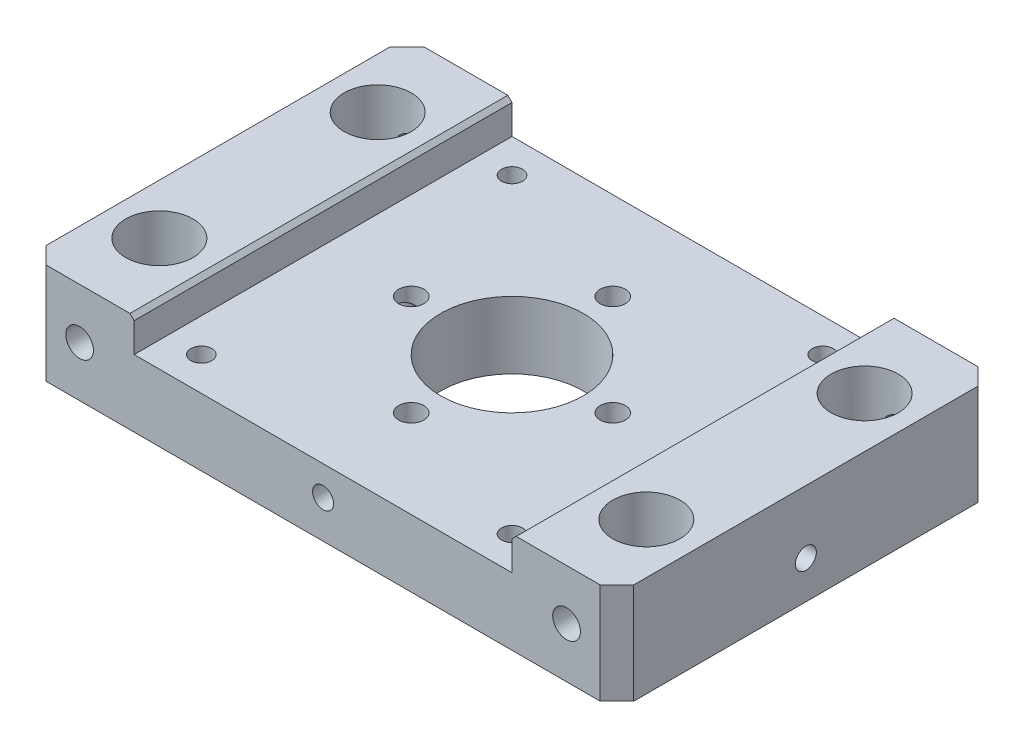
from build123d import *

# Parameters (mm, degrees)
SKETCH1_W                       = 70
SKETCH1_H                       = 45
BOSS_EXTRUDE1_DEPTH             = 12
SKETCH2_W                       = 45
SKETCH2_H                       = 45
CUT_EXTRUDE1_DEPTH              = 4
SKETCH3_R                       = 4
CUT_EXTRUDE2_DEPTH              = 50
SKETCH4_R                       = 8.5
CUT_EXTRUDE3_DEPTH              = 50
SKETCH5_R                       = 0.5
CUT_EXTRUDE4_DEPTH              = 7
M4_TAPPED_HOLE1_AT_2_COUNT      = 2
M4_TAPPED_HOLE1_AT_2_PITCH      = 58
SKETCH7_R                       = 1.5
CUT_EXTRUDE5_DEPTH              = 4.8
SKETCH8_R                       = 1.25
CUT_EXTRUDE6_DEPTH              = 23
CIRPATTERN1_COUNT               = 4
M3_TAPPED_HOLE4_D               = 2.5
M3_TAPPED_HOLE4_DEPTH           = 6
M3_TAPPED_HOLE4_TIP             = 0.751075774
M3_TAPPED_HOLE3_D               = 2.5
M3_TAPPED_HOLE3_DEPTH           = 7.5
M3_TAPPED_HOLE3_TIP             = 0.751075774
M3_TAPPED_HOLE3_ON_FACE_2_D     = 2.5
M3_TAPPED_HOLE3_ON_FACE_2_DEPTH = 7.5
M3_TAPPED_HOLE3_ON_FACE_2_TIP   = 0.751075774
CHAMFER1_SIZE                   = 0.5
M5_TAPPED_HOLE1_D               = 4.2
M5_TAPPED_HOLE1_DEPTH           = 10.4
M5_TAPPED_HOLE1_TIP             = 1.2618073
SKETCH13_R                      = 2
CUT_EXTRUDE8_DEPTH              = 24.5
CHAMFER2_SIZE                   = 2
M3_TAPPED_HOLE5_D               = 2.5
M3_TAPPED_HOLE6_D               = 2.5
M3_TAPPED_HOLE6_DEPTH           = 7.5
M3_TAPPED_HOLE6_TIP             = 0.751075774


with BuildPart() as part:
    # Sketch1 → Boss-Extrude1 (new body)
    with BuildSketch(Plane(origin=(0, 0, 0), x_dir=(1, 0, 0), z_dir=(0, 1, 0))):
        Rectangle(SKETCH1_W, SKETCH1_H)
    extrude(amount=BOSS_EXTRUDE1_DEPTH)

    # Sketch2 → Cut-Extrude1 (cut)
    with BuildSketch(Plane(origin=(0, 12, 0), x_dir=(1, 0, 0), z_dir=(0, 1, 0))):
        Rectangle(SKETCH2_W, SKETCH2_H)
    extrude(amount=-CUT_EXTRUDE1_DEPTH, mode=Mode.SUBTRACT)

    # Sketch3 → Cut-Extrude2 (cut)
    with BuildSketch(Plane(origin=(0, 12, 0), x_dir=(1, 0, 0), z_dir=(0, 1, 0))):
        with Locations(Location((-29, 13, 0), (0, 0, 270))):
            Circle(SKETCH3_R)
        with Locations(Location((-29, -13, 0), (0, 0, 270))):
            Circle(SKETCH3_R)
        with Locations(Location((29, -13, 0), (0, 0, 270))):
            Circle(SKETCH3_R)
        with Locations(Location((29, 13, 0), (0, 0, 270))):
            Circle(SKETCH3_R)
    extrude(amount=-CUT_EXTRUDE2_DEPTH, mode=Mode.SUBTRACT)

    # Sketch4 → Cut-Extrude3 (cut)
    with BuildSketch(Plane(origin=(0, 12, 0), x_dir=(1, 0, 0), z_dir=(0, 1, 0))):
        with Locations(Location((0, 0, 0), (0, 0, 270))):
            Circle(SKETCH4_R)
    extrude(amount=-CUT_EXTRUDE3_DEPTH, mode=Mode.SUBTRACT)

    # Sketch5 → Cut-Extrude4 (cut)
    with BuildSketch(Plane.XY.offset(22.5)):
        with Locations((-29, 6)):
            Circle(SKETCH5_R)
        with Locations(Location((29, 6, 0), (0, 0, 270))):
            Circle(SKETCH5_R)
    extrude(amount=-CUT_EXTRUDE4_DEPTH, mode=Mode.SUBTRACT)

    # Sketch6 → M4 Tapped Hole1 (revolve, cut)
    with BuildSketch(Plane(origin=(-29, 6, 22.5), x_dir=(0, -1, 0), z_dir=(1, 0, 0))):
        Polygon((0, 0), (0, 11.091420021), (1.65, 10.1), (1.65, 0), align=None)
    m4_tapped_hole1 = revolve(axis=Axis((-29, 6, 28.85), (0, 0, -1)), mode=Mode.SUBTRACT)

    # M4 Tapped Hole1 at 2: M4 Tapped Hole1 ×2
    with Locations(*[(i * M4_TAPPED_HOLE1_AT_2_PITCH, 0, 0) for i in range(1, M4_TAPPED_HOLE1_AT_2_COUNT)]):
        add(m4_tapped_hole1, mode=Mode.SUBTRACT)

    # Mirror1: M4 Tapped Hole1 across plane
    add(m4_tapped_hole1.mirror(Plane.XY), mode=Mode.SUBTRACT)

    # Mirror1 copy 1 sketch → Mirror1 copy 1 (revolve, cut)
    with BuildSketch(Plane(origin=(29, 6, -22.5), x_dir=(0, -1, 0), z_dir=(1, 0, 0))):
        Polygon((0, 0), (0, -11.091420021), (1.65, -10.1), (1.65, 0), align=None)
    revolve(axis=Axis((29, 6, -28.85), (0, 0, -1)), mode=Mode.SUBTRACT)

    # Sketch7 → Cut-Extrude5 (cut)
    with BuildSketch(Plane(origin=(0, 8, 0), x_dir=(1, 0, 0), z_dir=(0, 1, 0))):
        with Locations(Location((0, 12, 0), (0, 0, 270))):
            Circle(SKETCH7_R)
        with Locations(Location((12, 0, 0), (0, 0, 270))):
            Circle(SKETCH7_R)
        with Locations(Location((0, -12, 0), (0, 0, 270))):
            Circle(SKETCH7_R)
        with Locations(Location((-12, 0, 0), (0, 0, 270))):
            Circle(SKETCH7_R)
    extrude(amount=-CUT_EXTRUDE5_DEPTH, mode=Mode.SUBTRACT)

    # Sketch8 → Cut-Extrude6 (cut)
    with BuildSketch(Plane.ZY.offset(35)):
        with Locations((0, 4.5)):
            Circle(SKETCH8_R)
    cut_extrude6 = extrude(amount=-CUT_EXTRUDE6_DEPTH, mode=Mode.SUBTRACT)

    # CirPattern1: Cut-Extrude6 ×4 about axis
    cirpattern1_axis = Axis((0, -38, 0), (0, 1, 0))
    for i in range(1, CIRPATTERN1_COUNT):
        add(cut_extrude6.rotate(cirpattern1_axis, i * 360 / CIRPATTERN1_COUNT), mode=Mode.SUBTRACT)

    # M3 Tapped Hole4
    with Locations(Plane(origin=(35, 4.5, 0), x_dir=(0, 0, 1), z_dir=(1, 0, 0))):
        with Locations((0, 0)):
            Hole(M3_TAPPED_HOLE4_D / 2, depth=M3_TAPPED_HOLE4_DEPTH)
            with Locations((0, 0, -(M3_TAPPED_HOLE4_DEPTH + M3_TAPPED_HOLE4_TIP / 2))):  # 118° drill point
                Cone(0, M3_TAPPED_HOLE4_D / 2, M3_TAPPED_HOLE4_TIP, mode=Mode.SUBTRACT)

    # M3 Tapped Hole3
    with Locations(Plane(origin=(0, 4.5, 22.5), x_dir=(1, 0, 0), z_dir=(0, 0, 1))):
        with Locations((0, 0)):
            Hole(M3_TAPPED_HOLE3_D / 2, depth=M3_TAPPED_HOLE3_DEPTH)
            with Locations((0, 0, -(M3_TAPPED_HOLE3_DEPTH + M3_TAPPED_HOLE3_TIP / 2))):  # 118° drill point
                Cone(0, M3_TAPPED_HOLE3_D / 2, M3_TAPPED_HOLE3_TIP, mode=Mode.SUBTRACT)

    # M3 Tapped Hole3 on face 2
    with Locations(Plane(origin=(0, 4.5, -22.5), x_dir=(1, 0, 0), z_dir=(0, 0, 1))):
        with Locations((0, 0)):
            Hole(M3_TAPPED_HOLE3_ON_FACE_2_D / 2, depth=M3_TAPPED_HOLE3_ON_FACE_2_DEPTH)
            with Locations((0, 0, -(M3_TAPPED_HOLE3_ON_FACE_2_DEPTH + M3_TAPPED_HOLE3_ON_FACE_2_TIP / 2))):  # 118° drill point
                Cone(0, M3_TAPPED_HOLE3_ON_FACE_2_D / 2, M3_TAPPED_HOLE3_ON_FACE_2_TIP, mode=Mode.SUBTRACT)

    # Chamfer1
    chamfer1_edges = [part.edges().sort_by_distance(p)[0] for p in [
        (22.5, 12, 0),
        (-22.5, 12, 0),
    ]]
    chamfer(chamfer1_edges, length=CHAMFER1_SIZE)

    # M5 Tapped Hole1
    with Locations(Plane(origin=(-35, 4.5, 0), x_dir=(0, 0, -1), z_dir=(-1, 0, 0))):
        with Locations((0, 0)):
            Hole(M5_TAPPED_HOLE1_D / 2, depth=M5_TAPPED_HOLE1_DEPTH)
            with Locations((0, 0, -(M5_TAPPED_HOLE1_DEPTH + M5_TAPPED_HOLE1_TIP / 2))):  # 118° drill point
                Cone(0, M5_TAPPED_HOLE1_D / 2, M5_TAPPED_HOLE1_TIP, mode=Mode.SUBTRACT)

    # Sketch13 → Cut-Extrude8 (cut)
    with BuildSketch(Plane.ZY.offset(35)):
        with Locations((0, 4.5)):
            Circle(SKETCH13_R)
    extrude(amount=-CUT_EXTRUDE8_DEPTH, mode=Mode.SUBTRACT)

    # Chamfer2
    chamfer2_edges = [part.edges().sort_by_distance(p)[0] for p in [
        (35, 6, 22.5),
        (-35, 6, 22.5),
        (-35, 6, -22.5),
        (35, 6, -22.5),
    ]]
    chamfer(chamfer2_edges, length=CHAMFER2_SIZE)

    # M3 Tapped Hole5 (through all)
    with Locations(Plane(origin=(0, 8, 0), x_dir=(1, 0, 0), z_dir=(0, 1, 0))):
        with Locations((18.5, 18.5), (-18.5, 18.5), (-18.5, -18.5), (18.5, -18.5)):
            Hole(M3_TAPPED_HOLE5_D / 2)

    # M3 Tapped Hole6
    with Locations(Plane(origin=(0, 0, -22.5), x_dir=(-1, 0, 0), z_dir=(0, 0, -1))):
        with Locations((11.5, 5.5)):
            Hole(M3_TAPPED_HOLE6_D / 2, depth=M3_TAPPED_HOLE6_DEPTH)
            with Locations((0, 0, -(M3_TAPPED_HOLE6_DEPTH + M3_TAPPED_HOLE6_TIP / 2))):  # 118° drill point
                Cone(0, M3_TAPPED_HOLE6_D / 2, M3_TAPPED_HOLE6_TIP, mode=Mode.SUBTRACT)


solid = part.part
